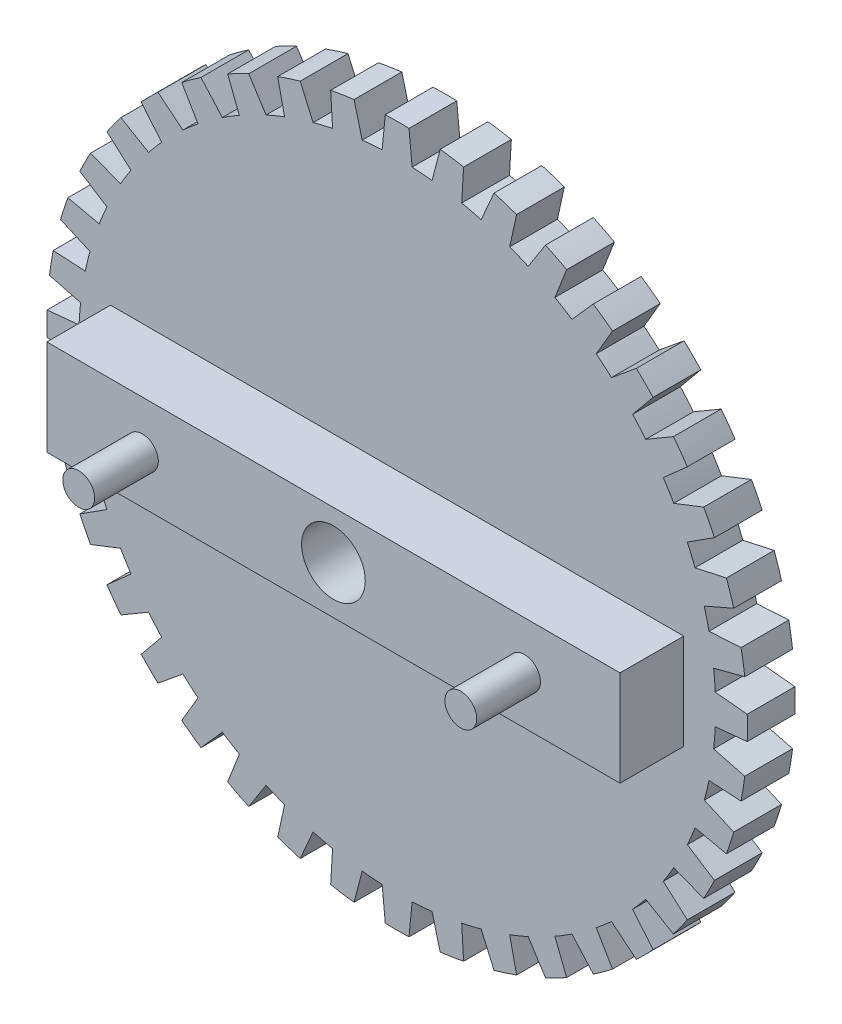
from build123d import *

# Parameters (mm, degrees)
SKETCH2_R           = 10
BOSS_EXTRUDE1_DEPTH = 15
SKETCH3_W           = 180
SKETCH3_H           = 30
SKETCH3_R           = 10
BOSS_EXTRUDE2_DEPTH = 20
SKETCH4_R           = 5
BOSS_EXTRUDE3_DEPTH = 20


with BuildPart() as part:
    # Sketch2 → Boss-Extrude1 (new body)
    with BuildSketch(Plane.XY):
        with BuildLine():
            Line((3.722086336, 189.93700957), (4.707648432, 179.889128769))
            ThreePointArc((4.707648432, 179.889128769), (7.845909573, 179.691733373), (10.976412955, 179.395766301))
            Line((10.976412955, 179.395766301), (13.521676003, 189.165765138))
            ThreePointArc((13.521676003, 189.165765138), (17.207791154, 188.645717465), (20.874198558, 188.001239968))
            Line((20.874198558, 188.001239968), (20.27579189, 177.922889373))
            ThreePointArc((20.27579189, 177.922889373), (23.344536386, 177.23699204), (26.390198626, 176.454950192))
            Line((26.390198626, 176.454950192), (30.432489804, 185.706497267))
            ThreePointArc((30.432489804, 185.706497267), (33.991869381, 184.616216792), (37.512318733, 183.406121402))
            Line((37.512318733, 183.406121402), (35.34467806, 173.545463454))
            ThreePointArc((35.34467806, 173.545463454), (38.268343237, 172.387953251), (41.154170022, 171.139093093))
            Line((41.154170022, 171.139093093), (46.593954705, 179.644384613))
            ThreePointArc((46.593954705, 179.644384613), (49.938954971, 178.010717661), (53.226761124, 176.264800941))
            Line((53.226761124, 176.264800941), (49.543260955, 166.864637765))
            ThreePointArc((49.543260955, 166.864637765), (52.249856472, 165.264016435), (54.90478917, 163.579089049))
            Line((54.90478917, 163.579089049), (61.608121806, 171.12869651))
            ThreePointArc((61.608121806, 171.12869651), (64.656377752, 168.991869381), (67.630584007, 166.753121597))
            Line((67.630584007, 166.753121597), (62.52192434, 158.044916406))
            ThreePointArc((62.52192434, 158.044916406), (64.944804833, 156.04059656), (67.30347019, 153.961090449))
            Line((67.30347019, 153.961090449), (75.105292482, 160.369117459))
            ThreePointArc((75.105292482, 160.369117459), (77.781745931, 157.781745931), (80.369117459, 155.105292482))
            Line((80.369117459, 155.105292482), (73.961090449, 147.30347019))
            ThreePointArc((73.961090449, 147.30347019), (76.04059656, 144.944804833), (78.044916406, 142.52192434))
            Line((78.044916406, 142.52192434), (86.753121597, 147.630584007))
            ThreePointArc((86.753121597, 147.630584007), (88.991869381, 144.656377752), (91.12869651, 141.608121806))
            Line((91.12869651, 141.608121806), (83.579089049, 134.90478917))
            ThreePointArc((83.579089049, 134.90478917), (85.264016435, 132.249856472), (86.864637765, 129.543260955))
            Line((86.864637765, 129.543260955), (96.264800941, 133.226761124))
            ThreePointArc((96.264800941, 133.226761124), (98.010717661, 129.938954971), (99.644384613, 126.593954705))
            Line((99.644384613, 126.593954705), (91.139093093, 121.154170022))
            ThreePointArc((91.139093093, 121.154170022), (92.387953251, 118.268343237), (93.545463454, 115.34467806))
            Line((93.545463454, 115.34467806), (103.406121402, 117.512318733))
            ThreePointArc((103.406121402, 117.512318733), (104.616216792, 113.991869381), (105.706497267, 110.432489804))
            Line((105.706497267, 110.432489804), (96.454950192, 106.390198626))
            ThreePointArc((96.454950192, 106.390198626), (97.23699204, 103.344536386), (97.922889373, 100.27579189))
            Line((97.922889373, 100.27579189), (108.001239968, 100.874198558))
            ThreePointArc((108.001239968, 100.874198558), (108.645717465, 97.207791154), (109.165765138, 93.521676003))
            Line((109.165765138, 93.521676003), (99.395766301, 90.976412955))
            ThreePointArc((99.395766301, 90.976412955), (99.691733373, 87.845909573), (99.889128769, 84.707648432))
            Line((99.889128769, 84.707648432), (109.93700957, 83.722086336))
            ThreePointArc((109.93700957, 83.722086336), (110, 80), (109.93700957, 76.277913664))
            Line((109.93700957, 76.277913664), (99.889128769, 75.292351568))
            ThreePointArc((99.889128769, 75.292351568), (99.691733373, 72.154090427), (99.395766301, 69.023587045))
            Line((99.395766301, 69.023587045), (109.165765138, 66.478323997))
            ThreePointArc((109.165765138, 66.478323997), (108.645717465, 62.792208846), (108.001239968, 59.125801442))
            Line((108.001239968, 59.125801442), (97.922889373, 59.72420811))
            ThreePointArc((97.922889373, 59.72420811), (97.23699204, 56.655463614), (96.454950192, 53.609801374))
            Line((96.454950192, 53.609801374), (105.706497267, 49.567510196))
            ThreePointArc((105.706497267, 49.567510196), (104.616216792, 46.008130619), (103.406121402, 42.487681267))
            Line((103.406121402, 42.487681267), (93.545463454, 44.65532194))
            ThreePointArc((93.545463454, 44.65532194), (92.387953251, 41.731656763), (91.139093093, 38.845829978))
            Line((91.139093093, 38.845829978), (99.644384613, 33.406045295))
            ThreePointArc((99.644384613, 33.406045295), (98.010717661, 30.061045029), (96.264800941, 26.773238876))
            Line((96.264800941, 26.773238876), (86.864637765, 30.456739045))
            ThreePointArc((86.864637765, 30.456739045), (85.264016435, 27.750143528), (83.579089049, 25.09521083))
            Line((83.579089049, 25.09521083), (91.12869651, 18.391878194))
            ThreePointArc((91.12869651, 18.391878194), (88.991869381, 15.343622248), (86.753121597, 12.369415993))
            Line((86.753121597, 12.369415993), (78.044916406, 17.47807566))
            ThreePointArc((78.044916406, 17.47807566), (76.04059656, 15.055195167), (73.961090449, 12.69652981))
            Line((73.961090449, 12.69652981), (80.369117459, 4.894707518))
            ThreePointArc((80.369117459, 4.894707518), (77.781745931, 2.218254069), (75.105292482, -0.369117459))
            Line((75.105292482, -0.369117459), (67.30347019, 6.038909551))
            ThreePointArc((67.30347019, 6.038909551), (64.944804833, 3.95940344), (62.52192434, 1.955083594))
            Line((62.52192434, 1.955083594), (67.630584007, -6.753121597))
            ThreePointArc((67.630584007, -6.753121597), (64.656377752, -8.991869381), (61.608121806, -11.12869651))
            Line((61.608121806, -11.12869651), (54.90478917, -3.579089049))
            ThreePointArc((54.90478917, -3.579089049), (52.249856472, -5.264016435), (49.543260955, -6.864637765))
            Line((49.543260955, -6.864637765), (53.226761124, -16.264800941))
            ThreePointArc((53.226761124, -16.264800941), (49.938954971, -18.010717661), (46.593954705, -19.644384613))
            Line((46.593954705, -19.644384613), (41.154170022, -11.139093093))
            ThreePointArc((41.154170022, -11.139093093), (38.268343237, -12.387953251), (35.34467806, -13.545463454))
            Line((35.34467806, -13.545463454), (37.512318733, -23.406121402))
            ThreePointArc((37.512318733, -23.406121402), (33.991869381, -24.616216792), (30.432489804, -25.706497267))
            Line((30.432489804, -25.706497267), (26.390198626, -16.454950192))
            ThreePointArc((26.390198626, -16.454950192), (23.344536386, -17.23699204), (20.27579189, -17.922889373))
            Line((20.27579189, -17.922889373), (20.874198558, -28.001239968))
            ThreePointArc((20.874198558, -28.001239968), (17.207791154, -28.645717465), (13.521676003, -29.165765138))
            Line((13.521676003, -29.165765138), (10.976412955, -19.395766301))
            ThreePointArc((10.976412955, -19.395766301), (7.845909573, -19.691733373), (4.707648432, -19.889128769))
            Line((4.707648432, -19.889128769), (3.722086336, -29.93700957))
            ThreePointArc((3.722086336, -29.93700957), (0, -30), (-3.722086336, -29.93700957))
            Line((-3.722086336, -29.93700957), (-4.707648432, -19.889128769))
            ThreePointArc((-4.707648432, -19.889128769), (-7.845909573, -19.691733373), (-10.976412955, -19.395766301))
            Line((-10.976412955, -19.395766301), (-13.521676003, -29.165765138))
            ThreePointArc((-13.521676003, -29.165765138), (-17.207791154, -28.645717465), (-20.874198558, -28.001239968))
            Line((-20.874198558, -28.001239968), (-20.27579189, -17.922889373))
            ThreePointArc((-20.27579189, -17.922889373), (-23.344536386, -17.23699204), (-26.390198626, -16.454950192))
            Line((-26.390198626, -16.454950192), (-30.432489804, -25.706497267))
            ThreePointArc((-30.432489804, -25.706497267), (-33.991869381, -24.616216792), (-37.512318733, -23.406121402))
            Line((-37.512318733, -23.406121402), (-35.34467806, -13.545463454))
            ThreePointArc((-35.34467806, -13.545463454), (-38.268343237, -12.387953251), (-41.154170022, -11.139093093))
            Line((-41.154170022, -11.139093093), (-46.593954705, -19.644384613))
            ThreePointArc((-46.593954705, -19.644384613), (-49.938954971, -18.010717661), (-53.226761124, -16.264800941))
            Line((-53.226761124, -16.264800941), (-49.543260955, -6.864637765))
            ThreePointArc((-49.543260955, -6.864637765), (-52.249856472, -5.264016435), (-54.90478917, -3.579089049))
            Line((-54.90478917, -3.579089049), (-61.608121806, -11.12869651))
            ThreePointArc((-61.608121806, -11.12869651), (-64.656377752, -8.991869381), (-67.630584007, -6.753121597))
            Line((-67.630584007, -6.753121597), (-62.52192434, 1.955083594))
            ThreePointArc((-62.52192434, 1.955083594), (-64.944804833, 3.95940344), (-67.30347019, 6.038909551))
            Line((-67.30347019, 6.038909551), (-75.105292482, -0.369117459))
            ThreePointArc((-75.105292482, -0.369117459), (-77.781745931, 2.218254069), (-80.369117459, 4.894707518))
            Line((-80.369117459, 4.894707518), (-73.961090449, 12.69652981))
            ThreePointArc((-73.961090449, 12.69652981), (-76.04059656, 15.055195167), (-78.044916406, 17.47807566))
            Line((-78.044916406, 17.47807566), (-86.753121597, 12.369415993))
            ThreePointArc((-86.753121597, 12.369415993), (-88.991869381, 15.343622248), (-91.12869651, 18.391878194))
            Line((-91.12869651, 18.391878194), (-83.579089049, 25.09521083))
            ThreePointArc((-83.579089049, 25.09521083), (-85.264016435, 27.750143528), (-86.864637765, 30.456739045))
            Line((-86.864637765, 30.456739045), (-96.264800941, 26.773238876))
            ThreePointArc((-96.264800941, 26.773238876), (-98.010717661, 30.061045029), (-99.644384613, 33.406045295))
            Line((-99.644384613, 33.406045295), (-91.139093093, 38.845829978))
            ThreePointArc((-91.139093093, 38.845829978), (-92.387953251, 41.731656763), (-93.545463454, 44.65532194))
            Line((-93.545463454, 44.65532194), (-103.406121402, 42.487681267))
            ThreePointArc((-103.406121402, 42.487681267), (-104.616216792, 46.008130619), (-105.706497267, 49.567510196))
            Line((-105.706497267, 49.567510196), (-96.454950192, 53.609801374))
            ThreePointArc((-96.454950192, 53.609801374), (-97.23699204, 56.655463614), (-97.922889373, 59.72420811))
            Line((-97.922889373, 59.72420811), (-108.001239968, 59.125801442))
            ThreePointArc((-108.001239968, 59.125801442), (-108.645717465, 62.792208846), (-109.165765138, 66.478323997))
            Line((-109.165765138, 66.478323997), (-99.395766301, 69.023587045))
            ThreePointArc((-99.395766301, 69.023587045), (-99.691733373, 72.154090427), (-99.889128769, 75.292351568))
            Line((-99.889128769, 75.292351568), (-109.93700957, 76.277913664))
            ThreePointArc((-109.93700957, 76.277913664), (-110, 80), (-109.93700957, 83.722086336))
            Line((-109.93700957, 83.722086336), (-99.889128769, 84.707648432))
            ThreePointArc((-99.889128769, 84.707648432), (-99.691733373, 87.845909573), (-99.395766301, 90.976412955))
            Line((-99.395766301, 90.976412955), (-109.165765138, 93.521676003))
            ThreePointArc((-109.165765138, 93.521676003), (-108.645717465, 97.207791154), (-108.001239968, 100.874198558))
            Line((-108.001239968, 100.874198558), (-97.922889373, 100.27579189))
            ThreePointArc((-97.922889373, 100.27579189), (-97.23699204, 103.344536386), (-96.454950192, 106.390198626))
            Line((-96.454950192, 106.390198626), (-105.706497267, 110.432489804))
            ThreePointArc((-105.706497267, 110.432489804), (-104.616216792, 113.991869381), (-103.406121402, 117.512318733))
            Line((-103.406121402, 117.512318733), (-93.545463454, 115.34467806))
            ThreePointArc((-93.545463454, 115.34467806), (-92.387953251, 118.268343237), (-91.139093093, 121.154170022))
            Line((-91.139093093, 121.154170022), (-99.644384613, 126.593954705))
            ThreePointArc((-99.644384613, 126.593954705), (-98.010717661, 129.938954971), (-96.264800941, 133.226761124))
            Line((-96.264800941, 133.226761124), (-86.864637765, 129.543260955))
            ThreePointArc((-86.864637765, 129.543260955), (-85.264016435, 132.249856472), (-83.579089049, 134.90478917))
            Line((-83.579089049, 134.90478917), (-91.12869651, 141.608121806))
            ThreePointArc((-91.12869651, 141.608121806), (-88.991869381, 144.656377752), (-86.753121597, 147.630584007))
            Line((-86.753121597, 147.630584007), (-78.044916406, 142.52192434))
            ThreePointArc((-78.044916406, 142.52192434), (-76.04059656, 144.944804833), (-73.961090449, 147.30347019))
            Line((-73.961090449, 147.30347019), (-80.369117459, 155.105292482))
            ThreePointArc((-80.369117459, 155.105292482), (-77.781745931, 157.781745931), (-75.105292482, 160.369117459))
            Line((-75.105292482, 160.369117459), (-67.30347019, 153.961090449))
            ThreePointArc((-67.30347019, 153.961090449), (-64.944804833, 156.04059656), (-62.52192434, 158.044916406))
            Line((-62.52192434, 158.044916406), (-67.630584007, 166.753121597))
            ThreePointArc((-67.630584007, 166.753121597), (-64.656377752, 168.991869381), (-61.608121806, 171.12869651))
            Line((-61.608121806, 171.12869651), (-54.90478917, 163.579089049))
            ThreePointArc((-54.90478917, 163.579089049), (-52.249856472, 165.264016435), (-49.543260955, 166.864637765))
            Line((-49.543260955, 166.864637765), (-53.226761124, 176.264800941))
            ThreePointArc((-53.226761124, 176.264800941), (-49.938954971, 178.010717661), (-46.593954705, 179.644384613))
            Line((-46.593954705, 179.644384613), (-41.154170022, 171.139093093))
            ThreePointArc((-41.154170022, 171.139093093), (-38.268343237, 172.387953251), (-35.34467806, 173.545463454))
            Line((-35.34467806, 173.545463454), (-37.512318733, 183.406121402))
            ThreePointArc((-37.512318733, 183.406121402), (-33.991869381, 184.616216792), (-30.432489804, 185.706497267))
            Line((-30.432489804, 185.706497267), (-26.390198626, 176.454950192))
            ThreePointArc((-26.390198626, 176.454950192), (-23.344536386, 177.23699204), (-20.27579189, 177.922889373))
            Line((-20.27579189, 177.922889373), (-20.874198558, 188.001239968))
            ThreePointArc((-20.874198558, 188.001239968), (-17.207791154, 188.645717465), (-13.521676003, 189.165765138))
            Line((-13.521676003, 189.165765138), (-10.976412955, 179.395766301))
            ThreePointArc((-10.976412955, 179.395766301), (-7.845909573, 179.691733373), (-4.707648432, 179.889128769))
            Line((-4.707648432, 179.889128769), (-3.722086336, 189.93700957))
            ThreePointArc((-3.722086336, 189.93700957), (0, 190), (3.722086336, 189.93700957))
        make_face()
        with Locations((0, 80)):
            Circle(SKETCH2_R, mode=Mode.SUBTRACT)
    extrude(amount=BOSS_EXTRUDE1_DEPTH)

    # Sketch3 → Boss-Extrude2 (add)
    with BuildSketch(Plane.XY.offset(15)):
        with Locations((0, 80)):
            Rectangle(SKETCH3_W, SKETCH3_H)
        with Locations((0, 80)):
            Circle(SKETCH3_R, mode=Mode.SUBTRACT)
    extrude(amount=BOSS_EXTRUDE2_DEPTH)

    # Sketch4 → Boss-Extrude3 (add)
    with BuildSketch(Plane.XY.offset(35)):
        with Locations((60, 80)):
            Circle(SKETCH4_R)
        with Locations(Location((-60, 80, 0), (0, 0, 180))):
            Circle(SKETCH4_R)
    extrude(amount=BOSS_EXTRUDE3_DEPTH)


solid = part.part
